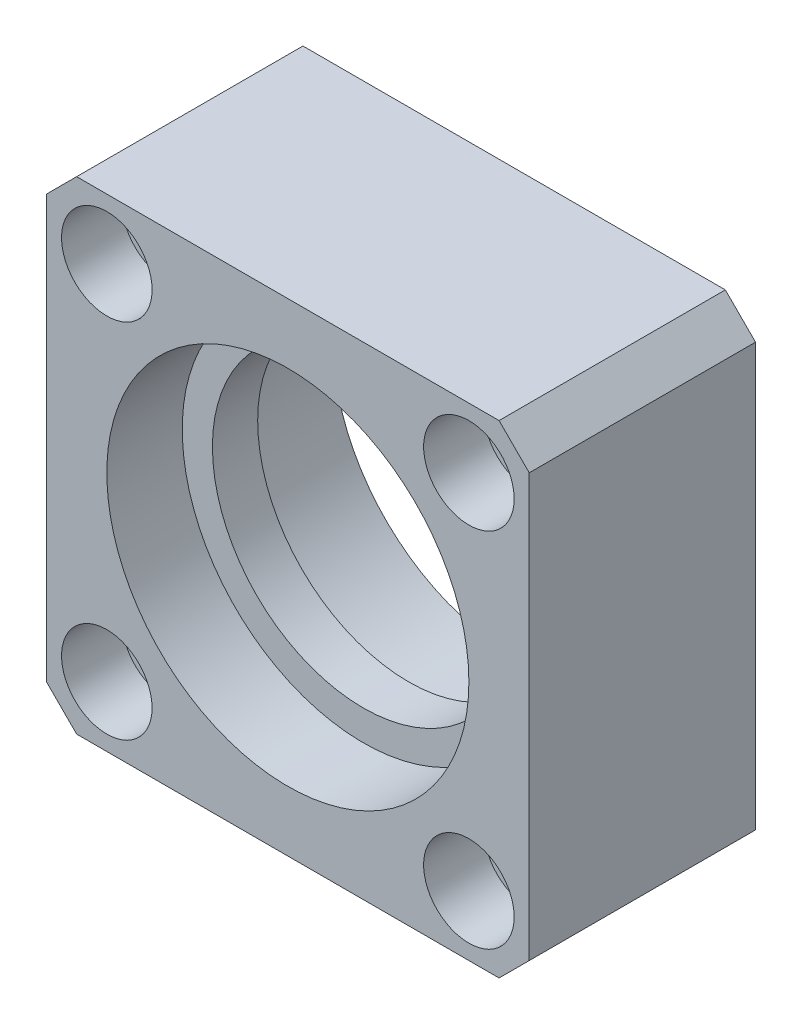
SolidWorks part; units mm, degrees
ref_plane "Front Plane" through (0, 0, 0) normal (0, 0, 1) x (1, 0, 0)
ref_plane "Top Plane" through (0, 0, 0) normal (0, 1, 0) x (1, 0, 0)
ref_plane "Right Plane" through (0, 0, 0) normal (1, 0, 0) x (0, 0, -1)
sketch "Sketch1" plane through (0, 0, 0) normal (0, 0, 1) x (1, 0, 0)
  line L1 (-16, 16) -> (16, 16)
  line L2 (-16, 16) -> (-16, -16)
  line L3 (-16, -16) -> (16, -16)
  line L4 (16, 16) -> (16, -16)
  line L5 (-16, 16) -> (16, -16) construction
  line L6 (-16, -16) -> (16, 16) construction
  point P0 (0, 0)
  dimension "D1" = 32
  dimension "D2" = 32
extrude "Boss-Extrude1" add sketch "Sketch1" along normal mid plane 15
sketch "Sketch2" plane through (0, 0, 7.5) normal (0, 0, 1) x (1, 0, 0)
  circle A0 centre (0, 0) radius 10
  dimension "D1" = 20
extrude "Cut-Extrude1" cut sketch "Sketch2" against normal through all
sketch "Sketch3" plane through (0, 0, 7.5) normal (0, 0, 1) x (1, 0, 0)
  circle A0 centre (0, 0) radius 12
  dimension "D1" = 24
extrude "Cut-Extrude2" cut sketch "Sketch3" against normal blind 5
sketch "Sketch4" plane through (0, 0, -7.5) normal (0, 0, -1) x (-1, 0, 0)
  circle A0 centre (0, 0) radius 12
  dimension "D1" = 24
extrude "Cut-Extrude3" cut sketch "Sketch4" against normal blind 7
chamfer "Chamfer1" distance 2 angle 45 4 edges at (-16, -16, 0) (16, -16, 0) (16, 16, 0) (-16, 16, 0)
hole_wizard "Hole size per socket head cap screw type1" positions "Sketch6" profile "Sketch5" counterbore size "M3" standard "Gb" end condition through all
sketch "Sketch6" plane through (0, 0, 7.5) normal (0, 0, 1) x (1, 0, 0)
  line L0 (0, 0) -> (0, 18.1224) construction
  line L2 (0, 0) -> (19.7825, 0) construction
  point P0 (-12, 12)
  point P2 (12, 12)
  point P4 (12, -12)
  point P6 (-12, -12)
  dimension "D1" = 24
  dimension "D2" = 24
sketch "Sketch5" plane through (-12, 12, 7.5) normal (1, 0, 0) x (0, -1, 0)
  line L0 (0, 0) -> (0, 15)
  line L1 (0, 15) -> (1.75, 15)
  line L3 (1.75, 15) -> (1.75, 4)
  line L4 (1.75, 4) -> (3, 4)
  line L5 (3, 4) -> (3, 0)
  line L7 (3, 0) -> (0, 0)
  line L11 (0, -6.35) -> (0, 107.95) construction
  dimension "通孔孔直径" = 3.5
  dimension "通孔孔深度" = 15
  dimension "柱形沉头孔直径" = 6
  dimension "柱形沉头孔深度" = 4
